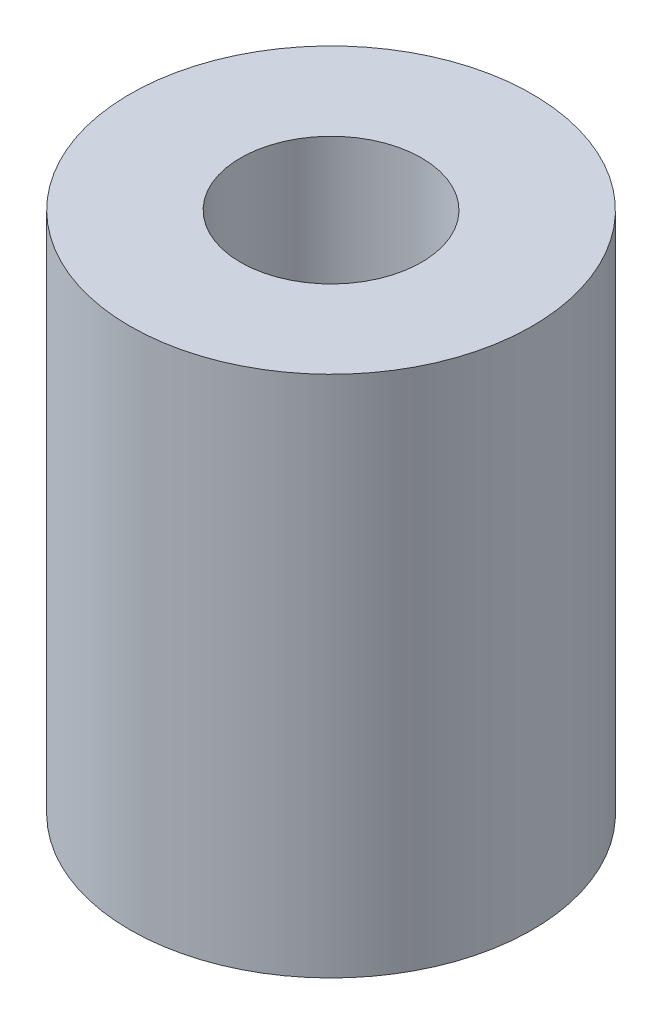
SolidWorks part; units mm, degrees
ref_plane "前视基准面" through (0, 0, 0) normal (0, 0, 1) x (1, 0, 0)
ref_plane "上视基准面" through (0, 0, 0) normal (0, 1, 0) x (1, 0, 0)
ref_plane "右视基准面" through (0, 0, 0) normal (1, 0, 0) x (0, 0, -1)
sketch "草图1" plane through (0, 0, 0) normal (0, 1, 0) x (1, 0, 0)
  circle A0 centre (0, 0) radius 22.5
  circle A1 centre (0, 0) radius 50
  dimension "D1" = 45
  dimension "D2" = 100
extrude "凸台-拉伸1" add sketch "草图1" along normal blind 130
